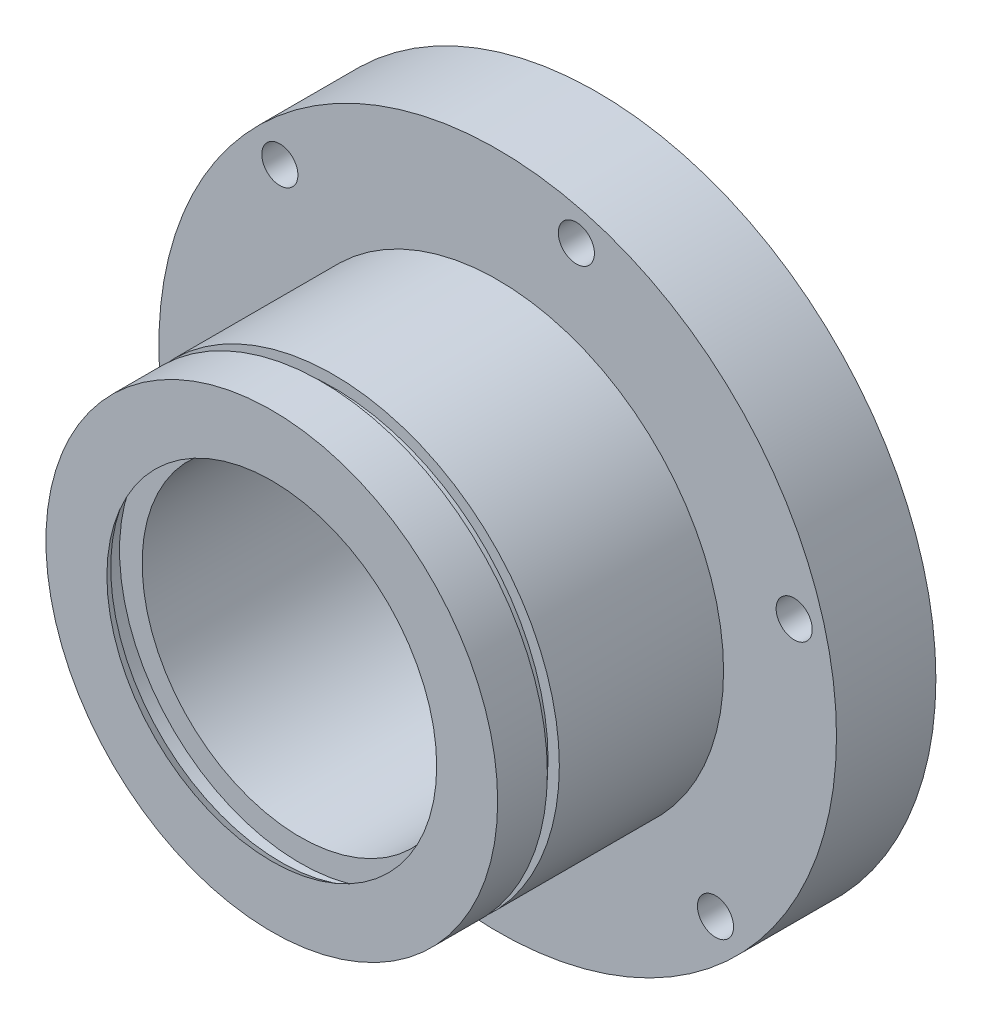
from build123d import *

# Parameters (mm, degrees)
SKETCH1_R           = 75
SKETCH1_R_2         = 35
BOSS_EXTRUDE1_DEPTH = 22
BOSS_EXTRUDE2_START = 22
SKETCH2_R           = 50
SKETCH2_R_2         = 35
BOSS_EXTRUDE2_DEPTH = 50
CUT_EXTRUDE1_START  = 58.35
SKETCH3_R           = 50
SKETCH3_R_2         = 47.5
CUT_EXTRUDE1_DEPTH  = 2.65
SKETCH5_R           = 4
CUT_EXTRUDE2_DEPTH  = 129.195163715
CHAMFER1_SIZE       = 1


with BuildPart() as part:
    # Sketch1 → Boss-Extrude1 (new body)
    with BuildSketch(Plane.XY):
        Circle(SKETCH1_R)
        Circle(SKETCH1_R_2, mode=Mode.SUBTRACT)
    extrude(amount=BOSS_EXTRUDE1_DEPTH)

    # Sketch2 → Boss-Extrude2 (add)
    with BuildSketch(Plane.XY.offset(BOSS_EXTRUDE2_START)):
        Circle(SKETCH2_R)
        Circle(SKETCH2_R_2, mode=Mode.SUBTRACT)
    extrude(amount=BOSS_EXTRUDE2_DEPTH)

    # Sketch3 → Cut-Extrude1 (cut)
    with BuildSketch(Plane.XY.offset(CUT_EXTRUDE1_START)):
        Circle(SKETCH3_R)
        Circle(SKETCH3_R_2, mode=Mode.SUBTRACT)
    extrude(amount=CUT_EXTRUDE1_DEPTH, mode=Mode.SUBTRACT)

    # Sketch5 → Cut-Extrude2 (cut, through all)
    with BuildSketch(Plane(origin=(0, 0, 0), x_dir=(-1, 0, 0), z_dir=(0, 0, -1))):
        with Locations((-17.413936667, 65.732448682)):
            Circle(SKETCH5_R)
        with Locations((48.219002079, 47.947135874)):
            Circle(SKETCH5_R)
        with Locations((65.632938745, -17.785312808)):
            Circle(SKETCH5_R)
        with Locations((17.413936667, -65.732448682)):
            Circle(SKETCH5_R)
        with Locations((-48.219002079, -47.947135874)):
            Circle(SKETCH5_R)
        with Locations((-65.632938745, 17.785312808)):
            Circle(SKETCH5_R)
    extrude(amount=-CUT_EXTRUDE2_DEPTH, mode=Mode.SUBTRACT)

    # Chamfer1
    chamfer1_edges = [part.edges().sort_by_distance(p)[0] for p in [
        (21.413936667, 65.732448682, 0),
        (-44.219002079, 47.947135874, 0),
        (-61.632938745, -17.785312808, 0),
        (-13.413936667, -65.732448682, 0),
        (52.219002079, -47.947135874, 0),
        (69.632938745, 17.785312808, 0),
    ]]
    chamfer(chamfer1_edges, length=CHAMFER1_SIZE)

    # Sketch7 → Cut-Revolve1 (revolve, cut)
    with BuildSketch(Plane(origin=(0, 0, 0), x_dir=(0, 0, -1), z_dir=(1, 0, 0)), mode=Mode.PRIVATE) as cut_revolve1_sk:
        Polygon((-72, 35), (-72, 36.5), (-70, 37.654700538), (-70, 40), (-65.7, 40), (-65.7, 35), align=None)
    revolve(cut_revolve1_sk.sketch.rotate(Axis((0, 0, 72), (0, 0, -1)), 90), axis=Axis((0, 0, 72), (0, 0, -1)), mode=Mode.SUBTRACT)


solid = part.part
